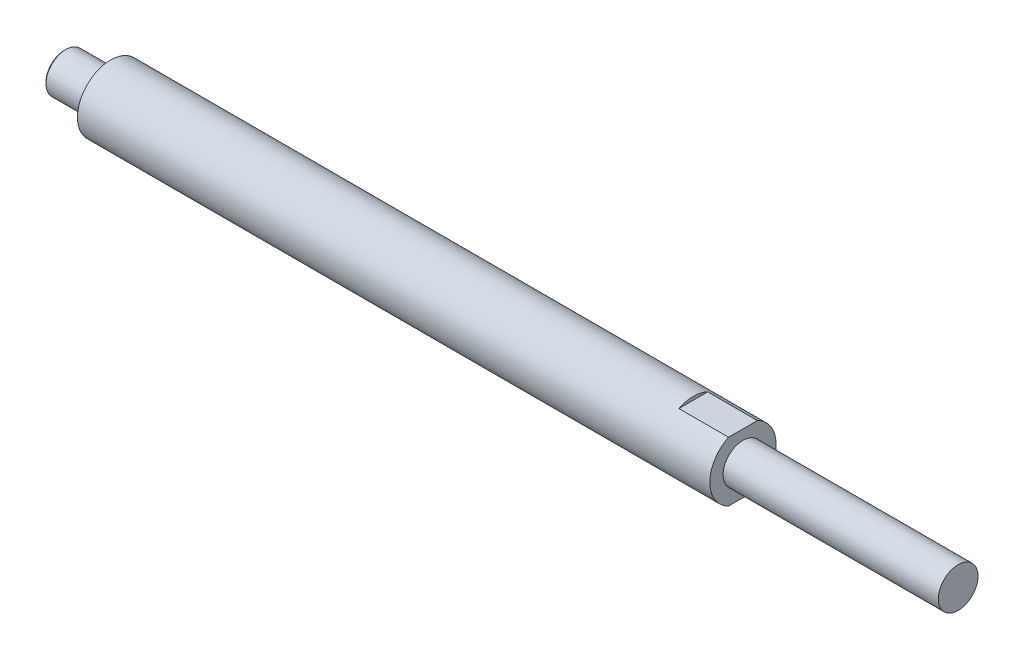
from build123d import *

# Parameters (mm, degrees)
SKETCH6_R           = 6
BOSS_EXTRUDE1_DEPTH = 14
CHAMFER1_SIZE       = 0.5
SKETCH7_W           = 15
SKETCH7_H           = 1
CUT_EXTRUDE1_DEPTH  = 10


with BuildPart() as part:
    # Sketch1 → Revolve1 (revolve)
    with BuildSketch(Plane.XY, mode=Mode.PRIVATE) as revolve1_sk:
        Polygon((0, 0), (0, 10), (191, 10), (191, 6), (256, 6), (256, 0), align=None)
    revolve(revolve1_sk.sketch.rotate(Axis((0, 0, 0), (1, 0, 0)), 90), axis=Axis((0, 0, 0), (1, 0, 0)))

    # Sketch6 → Boss-Extrude1 (add)
    with BuildSketch(Plane.ZY):
        Circle(SKETCH6_R)
    extrude(amount=BOSS_EXTRUDE1_DEPTH)

    # Chamfer1
    chamfer1_edges = [part.edges().sort_by_distance(p)[0] for p in [
        (-14, 0, -6),
    ]]
    chamfer(chamfer1_edges, length=CHAMFER1_SIZE)

    # Sketch7 → Cut-Extrude1 (cut, symmetric)
    with BuildSketch(Plane.XY):
        with Locations((183.5, 9.5)):
            Rectangle(SKETCH7_W, SKETCH7_H)
        with Locations((183.5, -9.5)):
            Rectangle(SKETCH7_W, SKETCH7_H)
    extrude(amount=CUT_EXTRUDE1_DEPTH, both=True, mode=Mode.SUBTRACT)


solid = part.part
